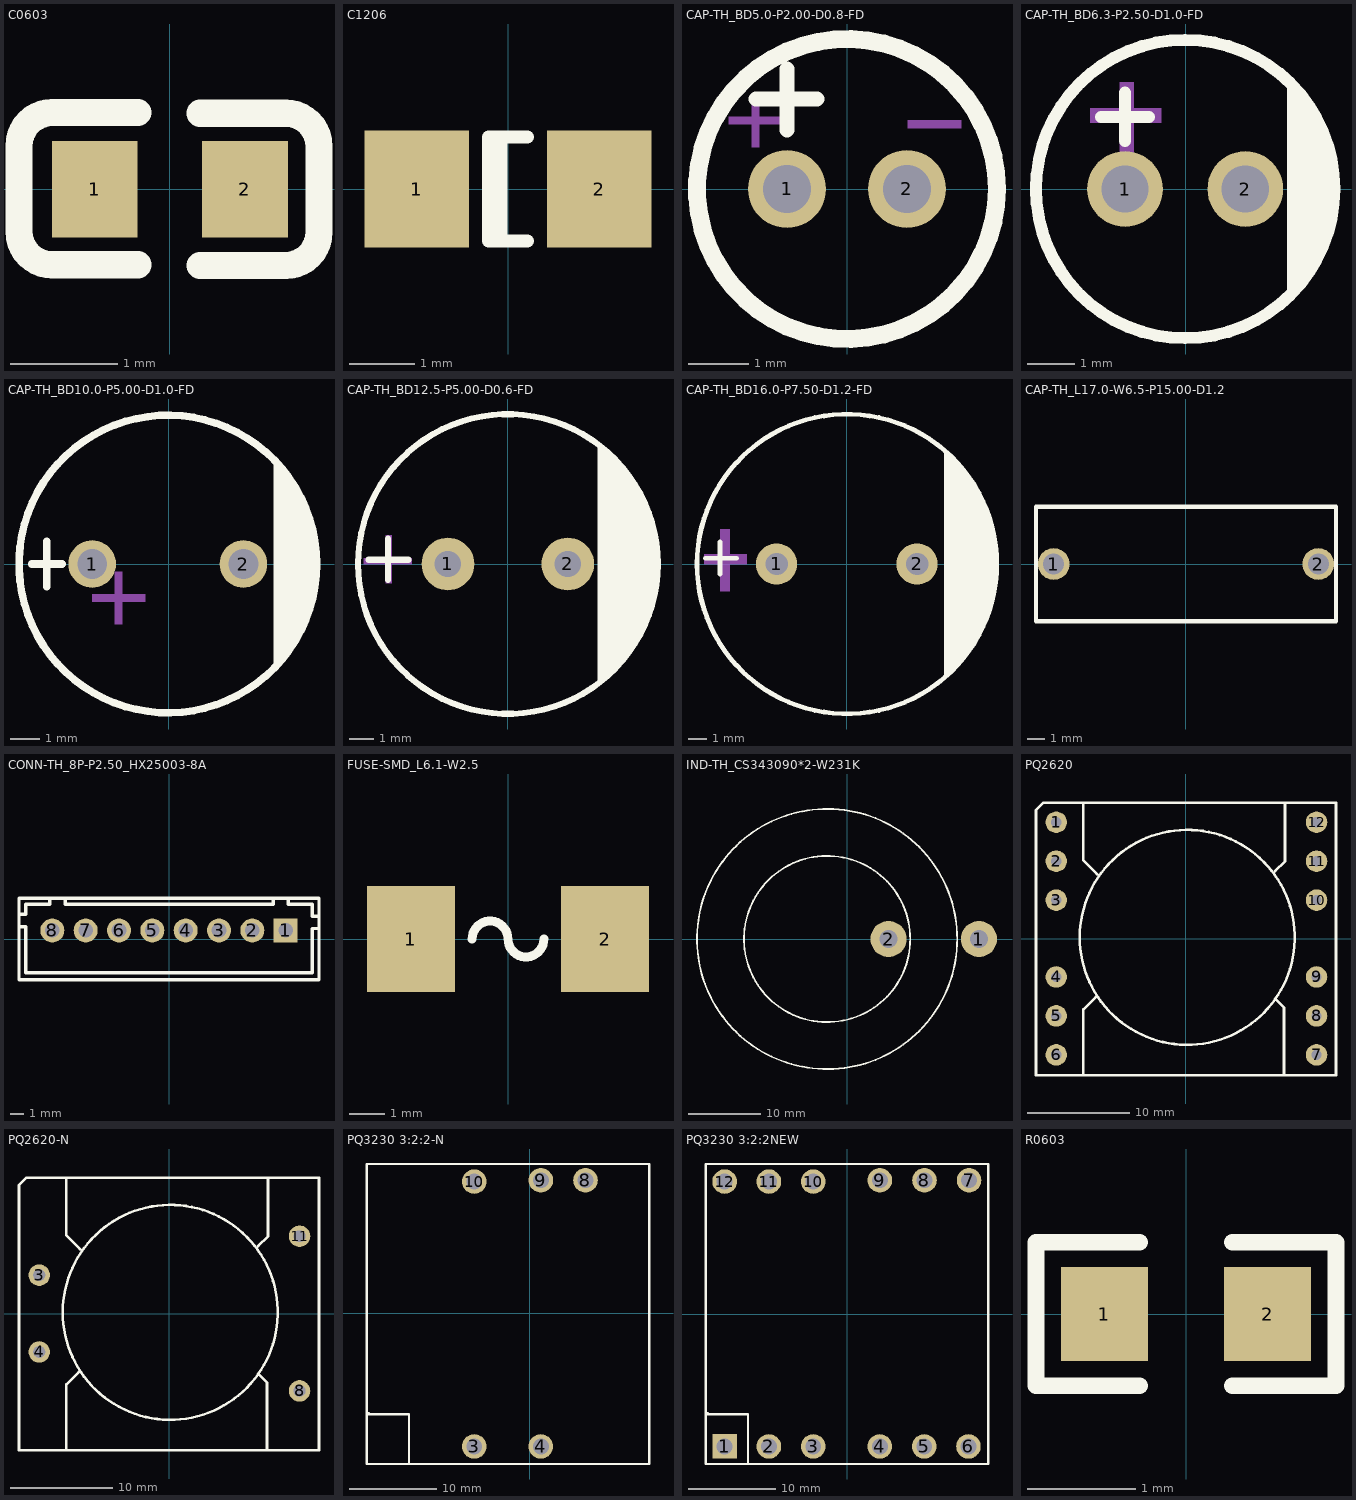
[diagram p0: the footprints below, top view; thin cyan lines are the x and y axes]
# Altium footprint library MISC89356.PcbLib: 29 footprints (part 1 of 2)
Each footprint in its own frame and in the unit in brackets; x right, y up, seen from the top. Pads: shape width x height; smd on the part's side, far side on the other; paste and mask are expansions set on the pad; w line width, h text height; cw(c..) or ccw(c..) is an arc to the next point about the centre after c.

## C0603 [mm]
pads (2):
  rect 0.8x0.9 smd: 1(-0.7,0) 2(0.7,0)
Top Overlay:
  lines w0.254: -0.296,-0.704 -1.096,-0.704 cw(c-1.096,-0.394) -1.406,-0.394 -1.405,0.406 cw(c-1.096,0.406) -1.096,0.715 -0.296,0.715 ; 0.28,-0.71 1.08,-0.71 ccw(c1.08,-0.4) 1.39,-0.4 1.39,0.4 ccw(c1.08,0.4) 1.08,0.71 0.28,0.71

## C1206 [mm] "Chip Capacitor; Body 3.2 x 1.6 mm (LxW typ)"
height 1.35
pads (2):
  rect 1.6x1.8 smd: 1(-1.4,0) 2(1.4,0)
Top Overlay:
  lines w0.2: -0.11,-0.8 -0.11,0.8 ; 0.3,-0.8 -0.3,-0.8 -0.3,0.8 0.3,0.8

## CAP-TH_BD5.0-P2.00-D0.8-FD [mm]
pads (2):
  round 1.3 hole 0.8: 1(-1,0) 2(1,0)
Top Overlay:
  circle w0.3: c0,0 r2.5
  lines w0.254: -1.516,1.5 -0.5,1.5 ; -1,0.984 -1,2
Mechanical 15:
  region: 1.016,1.143 1.905,1.143 1.905,1.016 1.016,1.016
  region: -1.588,0.699 -1.588,1.587 -1.461,1.587 -1.46,0.699
  region: -1.969,1.206 -1.08,1.206 -1.08,1.079 -1.969,1.079

## CAP-TH_BD6.3-P2.50-D1.0-FD [mm]
pads (2):
  round 1.6 hole 1: 1(-1.28,0) 2(1.26,0)
Top Overlay:
  circle w0.254: c-0.01,0 r3.15
  region: 2.15,2.287 2.27,2.184 2.585,1.816 2.838,1.402 3.023,0.955 3.136,0.483 3.175,0 3.136,-0.483 3.023,-0.955 2.838,-1.402 2.585,-1.816 2.27,-2.184 2.15,-2.287 2.149,-2.286
  lines w0.254: -1.788,1.524 -0.772,1.524 ; -1.28,1.016 -1.28,2.032
Mechanical 15:
  region: -1.391,0.752 -1.391,2.252 -1.091,2.252 -1.091,0.752
  region: -2.01,1.7 -0.51,1.7 -0.51,1.4 -2.01,1.4

## CAP-TH_BD10.0-P5.00-D1.0-FD [mm]
pads (2):
  round 1.6 hole 1: 1(-2.578,0) 2(2.502,0)
Top Overlay:
  circle w0.254: c-0.038,0 r5
  region: 3.518,3.556 3.518,-3.556 4.28,-2.54 4.788,-1.016 5.042,0.508 4.788,1.524
  lines w0.254: -4.61,0 -3.594,0 ; -4.102,-0.762 -4.102,0.762
Mechanical 15:
  region: -1.816,-2.032 -1.562,-2.032 -1.562,-0.254 -1.816,-0.254
  region: -2.578,-1.016 -0.8,-1.016 -0.8,-1.27 -2.578,-1.27

## CAP-TH_BD12.5-P5.00-D0.6-FD [mm]
pads (2):
  round 2.2 hole 1.1: 1(-2.5,0) 2(2.5,0)
Top Overlay:
  circle w0.254: c0,0 r6.25
  region: 3.75,5 3.75,-5 4.482,-4.268 4.489,-4.274 4.941,-3.769 5.333,-3.216 5.661,-2.623 5.92,-1.997 6.108,-1.345 6.221,-0.677 6.259,0 6.221,0.677 6.108,1.345 5.92,1.997 5.661,2.623 5.333,3.216 4.941,3.769 4.489,4.274 4.482,4.268
  lines w0.254: -5.817,0.178 -4.14,0.178 ; -5.004,-0.66 -5.004,1.067
Mechanical 15:
  region: -5.092,-0.811 -5.092,1.189 -4.842,1.189 -4.842,-0.811
  region: -6,0.25 -4,0.25 -4,0 -6,0

## CAP-TH_BD16.0-P7.50-D1.2-FD [mm]
pads (2):
  round 2.2 hole 1.2: 1(-3.751,0) 2(3.749,0)
Top Overlay:
  circle w0.254: c0,0 r8
  region: 5.207,-6.097 5.652,-5.699 6.255,-5.025 6.778,-4.288 7.215,-3.497 7.561,-2.662 7.811,-1.793 7.962,-0.902 8.013,0 7.962,0.902 7.811,1.793 7.561,2.662 7.215,3.497 6.778,4.288 6.255,5.025 5.652,5.699 5.207,6.097 5.206,6.096
  lines w0.254: -7.554,0.305 -5.877,0.305 ; -6.766,-0.533 -6.766,1.194
Mechanical 15:
  region: -7.621,0.508 -5.335,0.508 -5.335,0 -7.621,0
  region: -6.755,1.851 -6.247,1.851 -6.247,-1.451 -6.755,-1.451
  region: 7.699,-0.2 5.413,-0.2 5.413,0.308 7.699,0.308

## CAP-TH_L17.0-W6.5-P15.00-D1.2 [mm]
pads (2):
  round 1.8 hole 1.2: 1(-7.501,0) 2(7.501,0)
Top Overlay:
  lines w0.254: -8.5,-3.25 -8.5,3.25 8.5,3.25 8.5,-3.25 -8.5,-3.25

## CONN-TH_8P-P2.50_HX25003-8A [mm]
pads (8):
  rect 1.8x1.8 hole 1.1: 1(8.75,0.646)
  round 1.8 hole 1.1: 2(6.25,0.646) 3(3.75,0.646) 4(1.25,0.646) 5(-1.25,0.646) 6(-3.75,0.646) 7(-6.25,0.646) 8(-8.75,0.646)
Top Overlay:
  lines w0.254: -11.25,0.915 -10.75,0.915 -10.75,-2.521 10.749,-2.521 10.749,0.786 11.249,0.786 ; -11.25,1.845 -10.75,1.845 -10.75,2.604 -8.944,2.604 -8.944,3.054 ; -7.8,2.604 7.8,2.604 ; -7.793,2.601 -7.793,3.05 ; 7.807,2.601 7.807,3.05 ; 8.943,2.604 10.749,2.604 10.749,1.715 11.249,1.715 ; 8.95,2.602 8.95,3.05 ; -11.25,-3.054 -11.25,3.046 11.25,3.046 11.25,-3.054 -11.25,-3.054

## FUSE-SMD_L6.1-W2.5 [mm]
pads (2):
  rect 2.5x3 smd: 1(-2.75,0) 2(2.75,0)
Top Overlay:
  lines w0.254: -1.016,0 cw(c-0.508,0) 0,0 ccw(c0.508,0) 1.016,0

## IND-TH_CS343090*2-W231K [mm]
pads (2):
  round 5 hole 2.5: 1(18.25,0) 2(5.75,0)
Top Overlay:
  circle w0.254: c-2.75,0 r11.5
  circle w0.254: c-2.75,0 r18

## PQ2620 [mm]
pads (12):
  round 2.1 hole 1: 1(-12.662,11.395) 2(-12.662,7.595) 3(-12.662,3.795) 4(-12.662,-3.705) 5(-12.662,-7.505) 6(-12.662,-11.305) 7(12.738,-11.305) 8(12.738,-7.505) 9(12.738,-3.705) 10(12.738,3.795) 11(12.738,7.595)
  round 2.1 hole 1 slot 1.005 at 0 deg: 12(12.738,11.395)
Top Overlay:
  lines w0.254: -14.632,10.65 -14.632,12.585 ; -10.367,0.16 ccw(c0.12,0.162) -10.367,0.164 ; -10.022,-13.315 -10.022,-6.88 -8.782,-5.64 ; -10.022,13.3 -10.022,7.67 -8.687,6.335 ; 8.708,6.62 9.657,7.57 9.657,13.3 ; 8.803,-5.925 9.563,-6.685 9.563,-13.315 ; 14.637,13.315 14.637,-13.3 ; -14.632,12.585 -13.918,13.3 ; -14.632,12.585 -14.632,-13.31 -14.637,-13.315 14.623,-13.315 14.637,-13.3 ; -14.632,12.585 -13.918,13.3 ; -13.918,13.3 -13.917,13.3 ; -13.918,13.3 14.593,13.3 14.637,13.255 14.637,-13.3
Bottom Solder:
  lines w0.5: -13.956,-11.61 ccw(c-13.729,-11.61) -13.956,-11.605 ; -13.956,-7.81 ccw(c-13.729,-7.81) -13.956,-7.805 ; -13.956,-4.01 ccw(c-13.729,-4.01) -13.956,-4.005 ; -13.956,3.49 ccw(c-13.729,3.49) -13.956,3.495 ; -13.956,7.29 ccw(c-13.729,7.29) -13.956,7.295 ; -13.956,11.09 ccw(c-13.729,11.09) -13.956,11.095 ; -13.804,-10.695 ccw(c-13.577,-10.695) -13.804,-10.69 ; -13.804,-6.895 ccw(c-13.577,-6.895) -13.804,-6.89 ; -13.804,-3.095 ccw(c-13.577,-3.095) -13.804,-3.09 ; -13.804,4.405 ccw(c-13.577,4.405) -13.804,4.41 ; -13.804,8.205 ccw(c-13.577,8.205) -13.804,8.21 ; -13.804,12.005 ccw(c-13.577,12.005) -13.804,12.01 ; -13.283,-12.296 ccw(c-13.049,-12.296) -13.283,-12.29 ; -13.283,-8.496 ccw(c-13.049,-8.496) -13.283,-8.49 ; -13.283,-4.696 ccw(c-13.049,-4.696) -13.283,-4.69 ; -13.283,2.804 ccw(c-13.049,2.804) -13.283,2.81 ; -13.283,6.604 ccw(c-13.049,6.604) -13.283,6.61 ; -13.283,10.404 ccw(c-13.049,10.404) -13.283,10.41 ; -12.996,-10.213 ccw(c-12.766,-10.213) -12.995,-10.208 ; -12.996,-6.413 ccw(c-12.766,-6.413) -12.995,-6.408 ; -12.996,-2.613 ccw(c-12.766,-2.613) -12.995,-2.608 ; -12.996,4.887 ccw(c-12.766,4.887) -12.995,4.892 ; -12.996,8.687 ccw(c-12.766,8.687) -12.995,8.692 ; -12.996,12.487 ccw(c-12.766,12.487) -12.995,12.492 ; -12.363,-12.245 ccw(c-12.144,-12.245) -12.363,-12.24 ; -12.363,-8.445 ccw(c-12.144,-8.445) -12.363,-8.44 ; -12.363,-4.645 ccw(c-12.144,-4.645) -12.363,-4.64 ; -12.363,2.855 ccw(c-12.144,2.855) -12.363,2.86 ; -12.363,6.655 ccw(c-12.144,6.655) -12.363,6.66 ; -12.363,10.455 ccw(c-12.144,10.455) -12.363,10.46 ; -12.115,-10.543 ccw(c-11.881,-10.543) -12.115,-10.538 ; -12.115,-6.743 ccw(c-11.881,-6.743) -12.115,-6.738 ; -12.115,-2.943 ccw(c-11.881,-2.943) -12.115,-2.938 ; -12.115,4.557 ccw(c-11.881,4.557) -12.115,4.562 ; -12.115,8.357 ccw(c-11.881,8.357) -12.115,8.362 ; -12.115,12.157 ccw(c-11.881,12.157) -12.115,12.162 ; -11.85,-11.508 ccw(c-11.596,-11.508) -11.85,-11.503 ; -11.85,-7.708 ccw(c-11.596,-7.708) -11.85,-7.703 ; -11.85,-3.908 ccw(c-11.596,-3.908) -11.85,-3.903 ; -11.85,3.592 ccw(c-11.596,3.592) -11.85,3.597 ; -11.85,7.392 ccw(c-11.596,7.392) -11.85,7.397 ; -11.85,11.192 ccw(c-11.596,11.192) -11.85,11.197 ; 11.444,-11.61 ccw(c11.671,-11.61) 11.444,-11.605 ; 11.444,-7.81 ccw(c11.671,-7.81) 11.444,-7.805 ; 11.444,-4.01 ccw(c11.671,-4.01) 11.444,-4.005 ; 11.444,3.49 ccw(c11.671,3.49) 11.444,3.495 ; 11.444,7.29 ccw(c11.671,7.29) 11.444,7.295 ; 11.444,11.09 ccw(c11.671,11.09) 11.444,11.095 ; 11.596,-10.695 ccw(c11.823,-10.695) 11.596,-10.69 ; 11.596,-6.895 ccw(c11.823,-6.895) 11.596,-6.89 ; 11.596,-3.095 ccw(c11.823,-3.095) 11.596,-3.09 ; 11.596,4.405 ccw(c11.823,4.405) 11.596,4.41 ; 11.596,8.205 ccw(c11.823,8.205) 11.596,8.21 ; 11.596,12.005 ccw(c11.823,12.005) 11.596,12.01 ; 12.117,-12.296 ccw(c12.351,-12.296) 12.117,-12.29 ; 12.117,-8.496 ccw(c12.351,-8.496) 12.117,-8.49 ; 12.117,-4.696 ccw(c12.351,-4.696) 12.117,-4.69 ; 12.117,2.804 ccw(c12.351,2.804) 12.117,2.81 ; 12.117,6.604 ccw(c12.351,6.604) 12.117,6.61 ; 12.117,10.404 ccw(c12.351,10.404) 12.117,10.41 ; 12.404,-10.213 ccw(c12.634,-10.213) 12.405,-10.208 ; 12.404,-6.413 ccw(c12.634,-6.413) 12.405,-6.408 ; 12.404,-2.613 ccw(c12.634,-2.613) 12.405,-2.608 ; 12.404,4.887 ccw(c12.634,4.887) 12.405,4.892 ; 12.404,8.687 ccw(c12.634,8.687) 12.405,8.692 ; 12.404,12.487 ccw(c12.634,12.487) 12.405,12.492 ; 13.037,-12.245 ccw(c13.256,-12.245) 13.037,-12.24 ; 13.037,-8.445 ccw(c13.256,-8.445) 13.037,-8.44 ; 13.037,-4.645 ccw(c13.256,-4.645) 13.037,-4.64 ; 13.037,2.855 ccw(c13.256,2.855) 13.037,2.86 ; 13.037,6.655 ccw(c13.256,6.655) 13.037,6.66 ; 13.037,10.455 ccw(c13.256,10.455) 13.037,10.46 ; 13.285,-10.543 ccw(c13.519,-10.543) 13.285,-10.538 ; 13.285,-6.743 ccw(c13.519,-6.743) 13.285,-6.738 ; 13.285,-2.943 ccw(c13.519,-2.943) 13.285,-2.938 ; 13.285,4.557 ccw(c13.519,4.557) 13.285,4.562 ; 13.285,8.357 ccw(c13.519,8.357) 13.285,8.362 ; 13.285,12.157 ccw(c13.519,12.157) 13.285,12.162 ; 13.55,-11.508 ccw(c13.804,-11.508) 13.55,-11.503 ; 13.55,-7.708 ccw(c13.804,-7.708) 13.55,-7.703 ; 13.55,-3.908 ccw(c13.804,-3.908) 13.55,-3.903 ; 13.55,3.592 ccw(c13.804,3.592) 13.55,3.597 ; 13.55,7.392 ccw(c13.804,7.392) 13.55,7.397 ; 13.55,11.192 ccw(c13.804,11.192) 13.55,11.197

## PQ2620-N [mm]
pads (4):
  round 2.1 hole 1.1 slot 1.155 at 0 deg: 3(-12.7,3.75) 4(-12.7,-3.75) 8(12.7,-7.55) 11(12.7,7.55)
Top Overlay:
  lines w0.254: -14.67,10.605 -14.67,12.54 ; -10.405,0.115 ccw(c0.083,0.117) -10.405,0.119 ; -10.06,-13.36 -10.06,-6.925 -8.82,-5.685 ; -10.06,13.255 -10.06,7.625 -8.725,6.29 ; 8.67,6.575 9.62,7.525 9.62,13.255 ; 8.765,-5.97 9.525,-6.73 9.525,-13.36 ; 14.6,13.27 14.6,-13.345 ; -14.67,12.54 -13.955,13.255 ; -14.67,12.54 -14.67,-13.355 -14.675,-13.36 14.585,-13.36 14.6,-13.345 ; -14.67,12.54 -13.955,13.255 ; -13.955,13.255 14.555,13.255 14.6,13.21 14.6,-13.345 ; -13.955,13.255 -13.955,13.255
Bottom Solder:
  lines w0.5: -13.994,-4.055 ccw(c-13.767,-4.055) -13.994,-4.05 ; -13.994,3.445 ccw(c-13.767,3.445) -13.994,3.45 ; -13.842,-3.14 ccw(c-13.614,-3.14) -13.842,-3.135 ; -13.842,4.36 ccw(c-13.614,4.36) -13.842,4.365 ; -13.321,-4.741 ccw(c-13.087,-4.741) -13.321,-4.735 ; -13.321,2.759 ccw(c-13.087,2.759) -13.321,2.765 ; -13.033,-2.658 ccw(c-12.803,-2.658) -13.033,-2.653 ; -13.033,4.842 ccw(c-12.803,4.842) -13.033,4.847 ; -12.4,-4.69 ccw(c-12.182,-4.69) -12.4,-4.685 ; -12.4,2.81 ccw(c-12.182,2.81) -12.4,2.815 ; -12.152,-2.988 ccw(c-11.918,-2.988) -12.152,-2.983 ; -12.152,4.512 ccw(c-11.918,4.512) -12.152,4.517 ; -11.887,-3.953 ccw(c-11.633,-3.953) -11.887,-3.948 ; -11.887,3.547 ccw(c-11.633,3.547) -11.887,3.552 ; 11.406,-7.855 ccw(c11.633,-7.855) 11.406,-7.85 ; 11.406,7.245 ccw(c11.633,7.245) 11.406,7.25 ; 11.558,-6.94 ccw(c11.786,-6.94) 11.558,-6.935 ; 11.558,8.16 ccw(c11.786,8.16) 11.558,8.165 ; 12.079,-8.541 ccw(c12.313,-8.541) 12.079,-8.535 ; 12.079,6.559 ccw(c12.313,6.559) 12.079,6.565 ; 12.367,-6.458 ccw(c12.597,-6.458) 12.367,-6.453 ; 12.367,8.642 ccw(c12.597,8.642) 12.367,8.647 ; 13,-8.49 ccw(c13.218,-8.49) 13,-8.485 ; 13,6.61 ccw(c13.218,6.61) 13,6.615 ; 13.248,-6.788 ccw(c13.482,-6.788) 13.248,-6.783 ; 13.248,8.312 ccw(c13.482,8.312) 13.248,8.317 ; 13.513,-7.753 ccw(c13.767,-7.753) 13.513,-7.748 ; 13.513,7.347 ccw(c13.767,7.347) 13.513,7.352

## PQ3230 3:2:2-N [mm]
pads (5):
  round 2.8 hole 1.8: 3(-6.342,-15.17) 4(1.258,-15.17) 8(6.342,15.17) 9(1.262,15.17) 10(-6.342,15.03)
Top Overlay:
  lines w0.254: -18.364,-11.372 -18.364,-11.499 -13.787,-11.499 -13.787,-17.168 -12.141,-17.168 ; -18.59,-17.169 13.61,-17.169 13.61,17.031 -18.59,17.031 -18.59,-17.169

## PQ3230 3:2:2NEW [mm]
pads (12):
  rect 2.8x2.8 hole 1.8: 1(-13.952,-15.101)
  round 2.8 hole 1.8: 2(-8.902,-15.101) 3(-3.852,-15.101) 4(3.748,-15.101) 5(8.798,-15.101) 6(13.848,-15.101) 7(13.913,15.239) 8(8.833,15.239) 9(3.753,15.239) 10(-3.852,15.099) 11(-8.902,15.099) 12(-13.952,15.099)
Top Overlay:
  lines w0.254: -15.874,-11.303 -15.874,-11.43 -11.297,-11.43 -11.297,-17.1 -9.651,-17.1 ; -16.1,-17.1 -16.1,17.1 16.1,17.1 16.1,-17.1 -16.1,-17.1

## R0603 [mm]
pads (2):
  rect 0.806x0.864 smd: 1(-0.753,0) 2(0.753,0)
Top Overlay:
  lines w0.152: -0.426,-0.661 -1.385,-0.661 -1.385,0.661 -0.426,0.661 ; 0.426,-0.661 1.385,-0.661 1.385,0.661 0.426,0.661
Top Paste:
  region: -0.355,0.4 -0.355,0.172 -0.735,0.172 -0.735,-0.158 -0.355,-0.158 -0.355,-0.4 -0.405,-0.45 -1.195,-0.45 -1.245,-0.4 -1.245,0.4 -1.195,0.45 -0.405,0.45
  region: 1.195,0.45 0.395,0.45 0.345,0.4 0.345,0.172 0.715,0.172 0.715,-0.158 0.345,-0.158 0.345,-0.4 0.395,-0.45 1.195,-0.45 1.245,-0.4 1.245,0.4